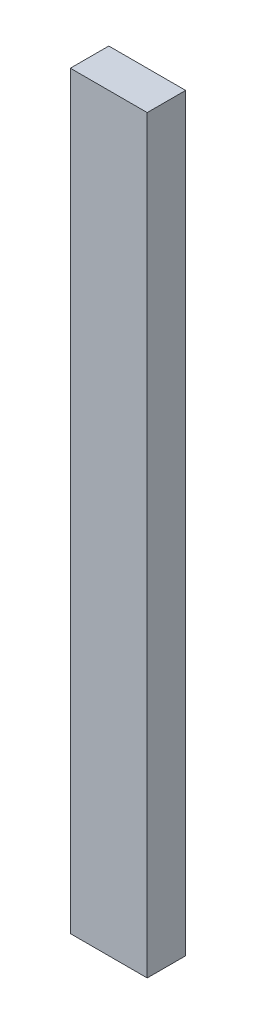
SolidWorks part; units mm, degrees
ref_plane "前视基准面" through (0, 0, 0) normal (0, 0, 1) x (1, 0, 0)
ref_plane "上视基准面" through (0, 0, 0) normal (0, 1, 0) x (1, 0, 0)
ref_plane "右视基准面" through (0, 0, 0) normal (1, 0, 0) x (0, 0, -1)
sketch "草图1" plane through (0, 0, 0) normal (0, 0, 1) x (1, 0, 0)
  line L1 (-10, -97.5) -> (10, -97.5)
  line L2 (-10, -97.5) -> (-10, 97.5)
  line L3 (-10, 97.5) -> (10, 97.5)
  line L4 (10, -97.5) -> (10, 97.5)
  line L5 (-10, -97.5) -> (10, 97.5) construction
  line L6 (-10, 97.5) -> (10, -97.5) construction
  point P0 (0, 0)
  dimension "D1" = 195
  dimension "D2" = 20
extrude "凸台-拉伸1" add sketch "草图1" along normal blind 10
